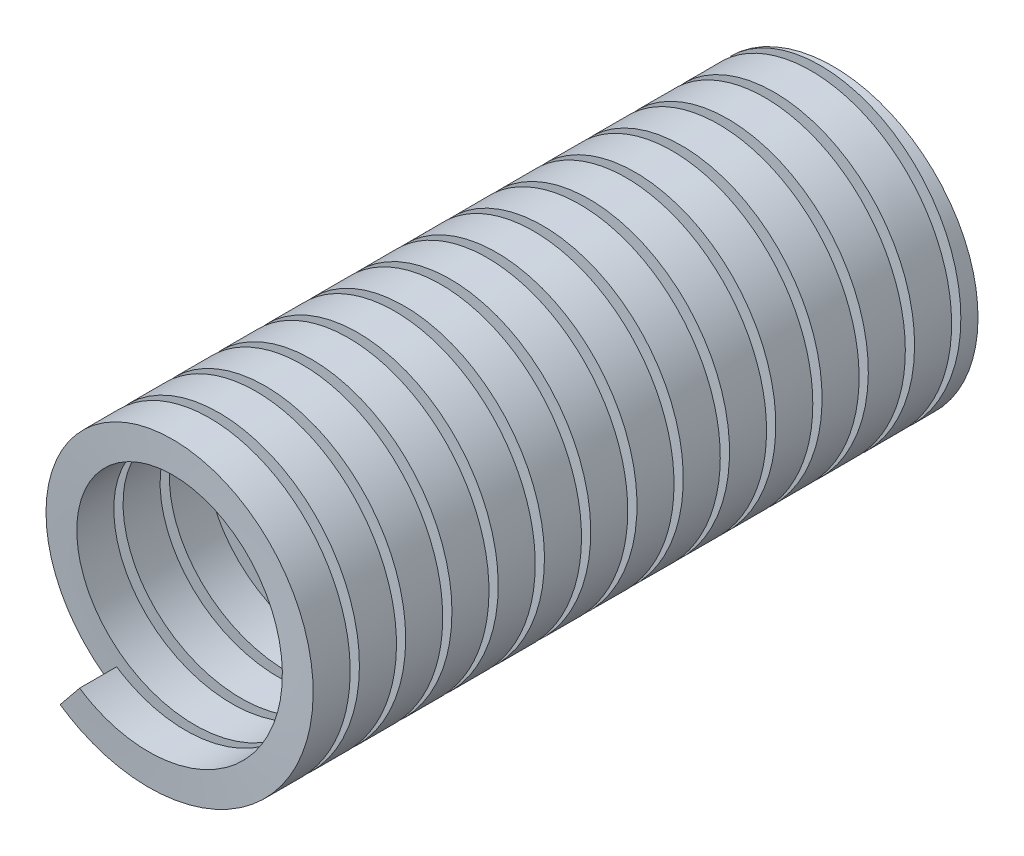
from build123d import *

# Parameters (mm, degrees)
SWEEP1_PITCH       = 15
SWEEP1_HEIGHT      = 221
SWEEP1_RADIUS      = 47
SWEEP1_START_ANGLE = 135
SKETCH5_W          = 10
SKETCH5_H          = 12
SKETCH7_R          = 75
CUT_EXTRUDE1_DEPTH = 60
SKETCH9_W          = 10
SKETCH9_H          = 8
CUT_EXTRUDE2_DEPTH = 55


with BuildPart() as part:
    # Sweep1: sweep along a helix
    with BuildLine() as sweep1_path:
        add(Helix(SWEEP1_PITCH, SWEEP1_HEIGHT, SWEEP1_RADIUS, center=(0, 0, 0), direction=(0, 0, 1), lefthand=True, mode=Mode.PRIVATE).rotate(Axis((0, 0, 0), (0, 0, 1)), SWEEP1_START_ANGLE))
    # Sketch5 → Sweep1 (sweep)
    with BuildSketch(Plane(origin=(0, 0, 0), x_dir=(1, 0, 0), z_dir=(0, 1, 0))):
        with Locations((41.999968696, -209.625000475)):
            Rectangle(SKETCH5_W, SKETCH5_H)
    sweep(path=sweep1_path.line, is_frenet=True)

    # Sketch7 → Cut-Extrude1 (cut)
    with BuildSketch(Plane.XY):
        Circle(SKETCH7_R)
    extrude(amount=-CUT_EXTRUDE1_DEPTH, mode=Mode.SUBTRACT)

    # Sketch9 → Cut-Extrude2 (cut)
    with BuildSketch(Plane.XY):
        with Locations((0, -36.3)):
            Rectangle(SKETCH9_W, SKETCH9_H)
    extrude(amount=CUT_EXTRUDE2_DEPTH, mode=Mode.SUBTRACT)


solid = part.part
